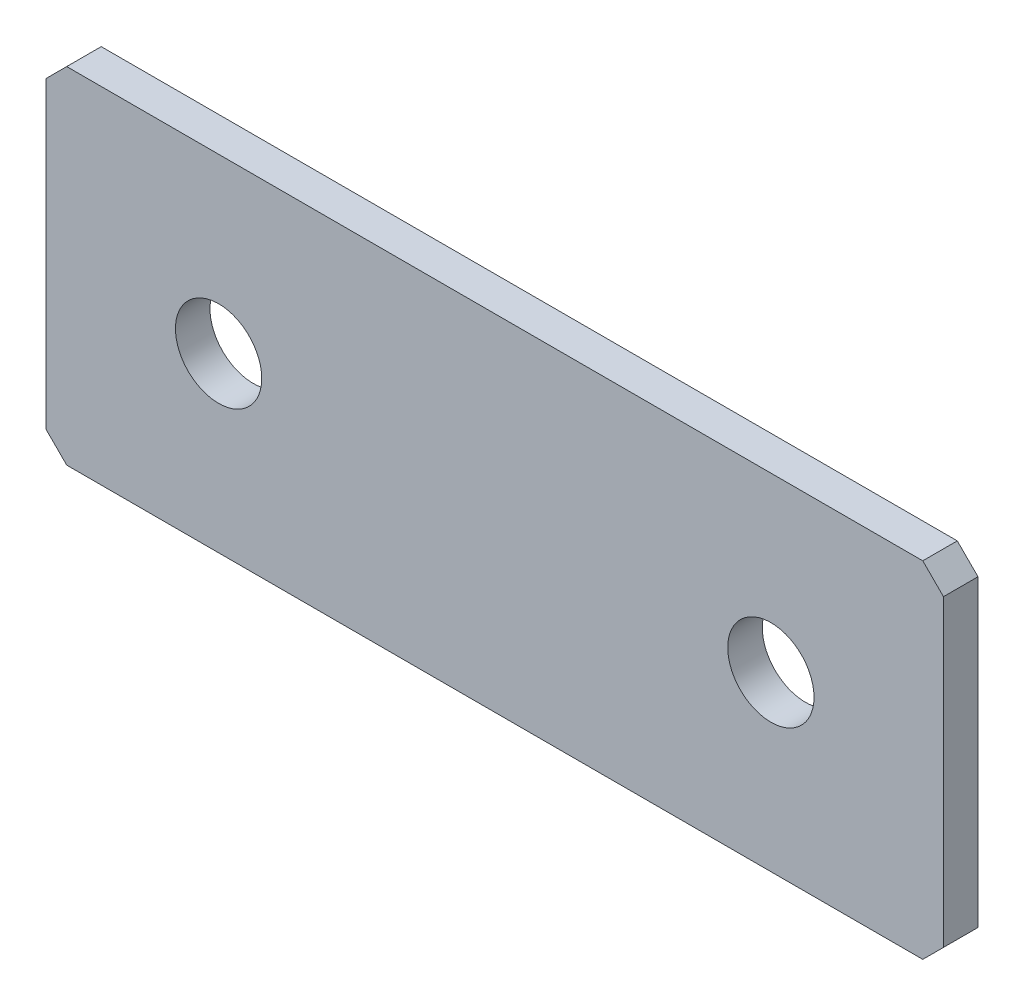
SolidWorks part; units mm, degrees
material "1023 碳钢板 (SS)"
ref_plane "Front Plane" through (0, 0, 0) normal (0, 0, 1) x (1, 0, 0)
ref_plane "Top Plane" through (0, 0, 0) normal (0, 1, 0) x (1, 0, 0)
ref_plane "Right Plane" through (0, 0, 0) normal (1, 0, 0) x (0, 0, -1)
ref_plane "Plane4" through (0, 0, 2.5) normal (0, 0, 1) x (1, 0, 0)
sketch "Sketch1" plane through (0, 0, 2.5) normal (0, 0, 1) x (1, 0, 0)
  line L0 (-62, -25) -> (62, -25)
  line L1 (62, -25) -> (65, -22)
  line L2 (65, -22) -> (65, 22)
  line L3 (65, 22) -> (62, 25)
  line L4 (62, 25) -> (-62, 25)
  line L5 (-62, 25) -> (-65, 22)
  line L6 (-65, 22) -> (-65, -22)
  line L7 (-65, -22) -> (-62, -25)
  circle A0 centre (-40, 0) radius 6.25
  circle A1 centre (40, 0) radius 6.25
extrude "Boss-Extrude1" add sketch "Sketch1" against normal blind 5
